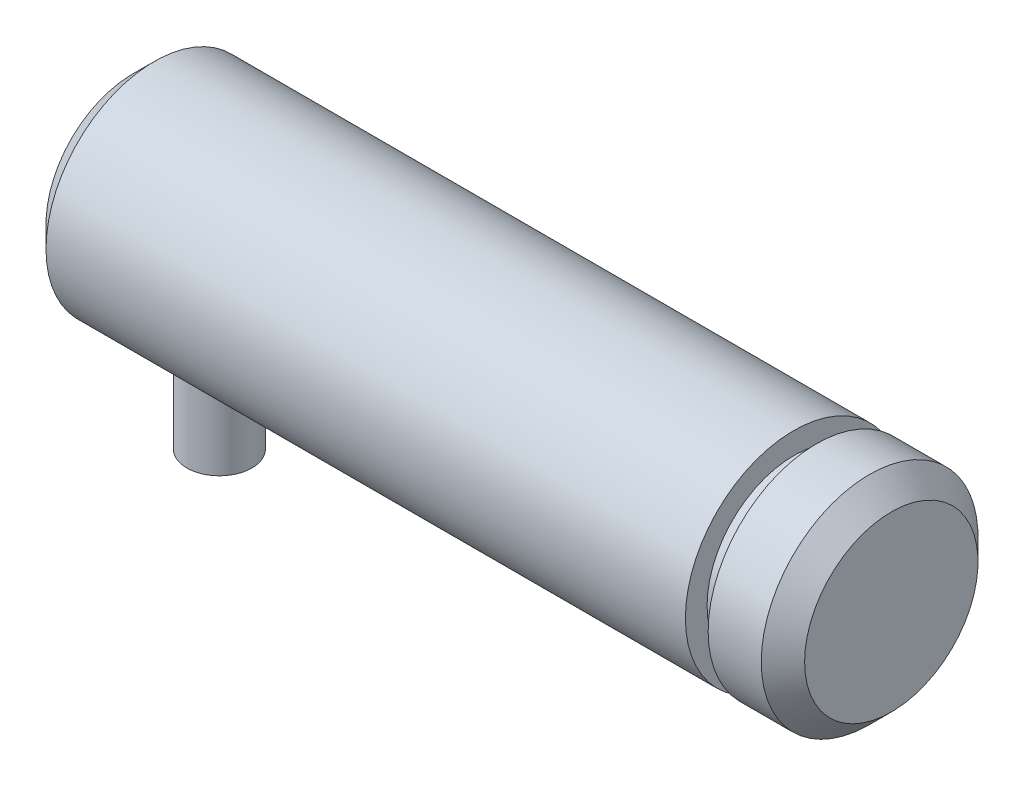
from build123d import *

# Parameters (mm, degrees)
SKETCH_2_W     = 1.5
SKETCH_2_H     = 4.230303993
CHAMFER_1_SIZE = 1


with BuildPart() as part:
    # 草图1 → 旋转1 (revolve)
    with BuildSketch(Plane(origin=(0, 0, 0), x_dir=(-1, 0, 0), z_dir=(0, 0, -1)), mode=Mode.PRIVATE) as revolve_1_sk:
        Polygon((-17.5, 5), (-17.5, 0), (17.5, 0), (17.5, 5), (-13, 5), (-13, 4), (-14.05, 4), (-14.05, 5), align=None)
    revolve(revolve_1_sk.sketch.rotate(Axis((17.5, 0, 0), (-1, 0, 0)), 270), axis=Axis((17.5, 0, 0), (-1, 0, 0)))

    # 草图2 → 旋转2 (revolve)
    with BuildSketch(Plane(origin=(-13.5, 0, 0), x_dir=(0, 0, -1), z_dir=(1, 0, 0))):
        with Locations((0.75, -6.884848004)):
            Rectangle(SKETCH_2_W, SKETCH_2_H)
    revolve(axis=Axis((-13.5, -4.769696007, 0), (0, -1, 0)))

    # 倒角1
    chamfer_1_edges = [part.edges().sort_by_distance(p)[0] for p in [
        (17.5, 0, -5),
        (-17.5, 0, -5),
    ]]
    chamfer(chamfer_1_edges, length=CHAMFER_1_SIZE)


solid = part.part
